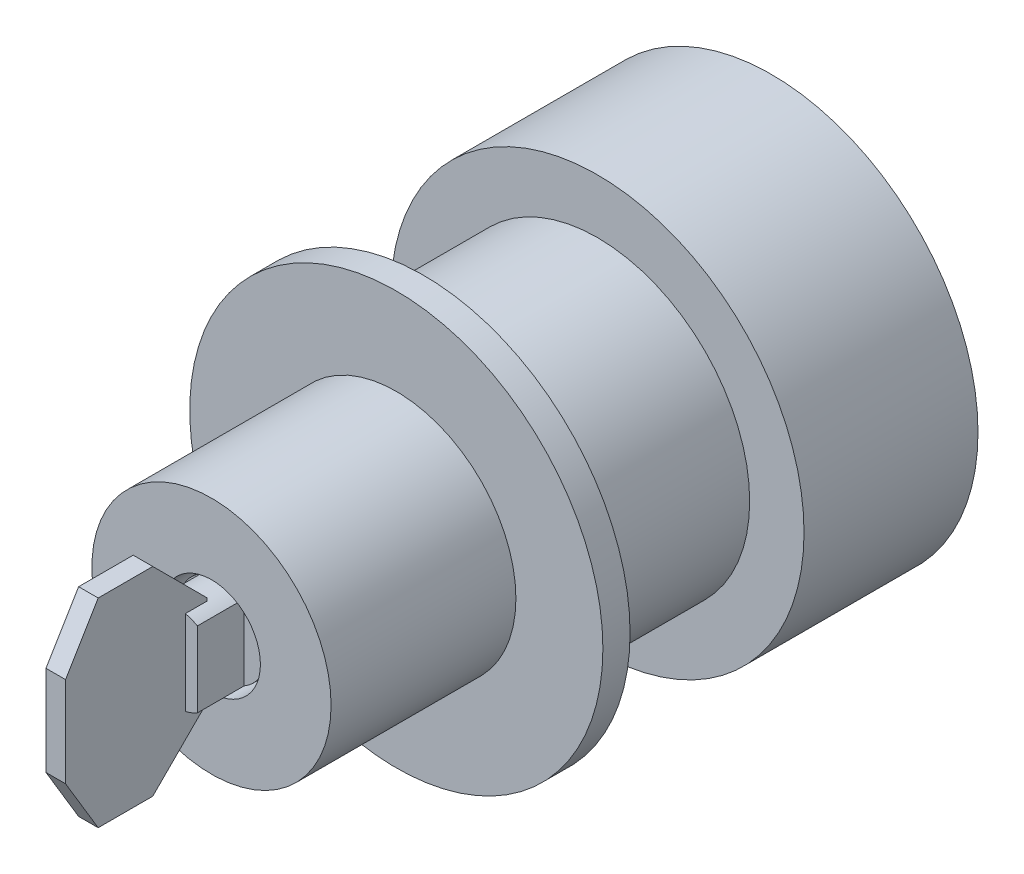
SolidWorks part; units mm, degrees
material "普通碳钢"
ref_plane "前视基准面" through (0, 0, 0) normal (0, 0, 1) x (1, 0, 0)
ref_plane "上视基准面" through (0, 0, 0) normal (0, 1, 0) x (1, 0, 0)
ref_plane "右视基准面" through (0, 0, 0) normal (1, 0, 0) x (0, 0, -1)
sketch "草图1" plane through (0, 0, 0) normal (0, 0, 1) x (1, 0, 0)
  circle A0 centre (0, 0) radius 19
extrude "拉伸1" add sketch "草图1" along normal blind 16
sketch "草图3" plane through (0, 0, 16) normal (0, 0, 1) x (1, 0, 0)
  circle A0 centre (0, 0) radius 14
extrude "拉伸2" add sketch "草图3" along normal blind 16
sketch "草图4" plane through (0, 0, 32) normal (0, 0, 1) x (1, 0, 0)
  circle A0 centre (0, 0) radius 19
extrude "拉伸3" add sketch "草图4" along normal blind 2.5
sketch "草图5" plane through (0, 0, 34.5) normal (0, 0, 1) x (1, 0, 0)
  circle A0 centre (0, 0) radius 11
extrude "拉伸4" add sketch "草图5" along normal blind 17
hole_wizard "孔1" positions "3D草图1" profile "草图6" legacy
sketch3d "3D草图1"
  point P0 (0, 0, 51.5)
sketch "草图6" plane through (0, 0, 51.5) normal (1, 0, 0) x (0, -1, 0)
  line L0 (0, 0) -> (0, 5)
  line L1 (0, 5) -> (4.5, 5)
  line L2 (4.5, 5) -> (4.5, 0)
  line L3 (4.5, 0) -> (0, 0)
  line L4 (0, 110) -> (0, -10) construction
  dimension "眻噤" = 9
  dimension "旮僅" = 5
sketch "草图7" plane through (0, 0, 46.5) normal (0, 0, 1) x (1, 0, 0)
  circle A0 centre (0, 0) radius 4
extrude "拉伸5" add sketch "草图7" along normal blind 4
sketch "草图9" plane through (0, 0, 50.5) normal (0, 0, 1) x (1, 0, 0)
  line L0 (-2, 3.4641) -> (-2, -3.4641)
  line L1 (2, 3.4641) -> (2, -3.4641)
  arc A1 (2, 3.4641) -> (-2, 3.4641) centre (0, 0) ccw
  circle A2 centre (0, 0) radius 4
  arc A3 (-2, -3.4641) -> (2, -3.4641) centre (0, 0) ccw
  dimension "D1" = 0
extrude "拉伸6" add sketch "草图9" along normal blind 4.3
sketch "草图10" plane through (0, 0, 54.8) normal (0, 0, 1) x (1, 0, 0)
  line L0 (-0.9, 3.8974) -> (-0.9, -3.8974)
  line L1 (0.9, 3.8974) -> (0.9, -3.8974)
  arc A0 (2, 3.4641) -> (-2, 3.4641) centre (0, 0) ccw construction
  arc A1 (0.9, 3.8974) -> (-0.9, 3.8974) centre (0, 0) ccw
  arc A2 (-2, -3.4641) -> (2, -3.4641) centre (0, 0) ccw construction
  arc A3 (-0.9, -3.8974) -> (0.9, -3.8974) centre (0, 0) ccw
extrude "切除-拉伸1" cut sketch "草图10" against normal blind 2
sketch "草图11" plane through (0, 0, 52.8) normal (0, 0, 1) x (1, 0, 0)
  line L0 (-0.9, 9.15) -> (-0.9, -9.15)
  line L1 (-0.9, 9.15) -> (0.9, 9.15)
  line L2 (0.9, 9.15) -> (0.9, -9.15)
  line L4 (0.9, -9.15) -> (-0.9, -9.15)
  dimension "D1" = 18.3
  dimension "D2" = 1.8
extrude "拉伸7" add sketch "草图11" along normal blind 13.02
chamfer "倒角1" distance 3 distance2 5 2 edges at (0, -9.15, 65.82) (0, 9.15, 65.82)
chamfer "倒角2" distance 5 distance2 5 2 edges at (0, -9.15, 52.8) (0, 9.15, 52.8)
